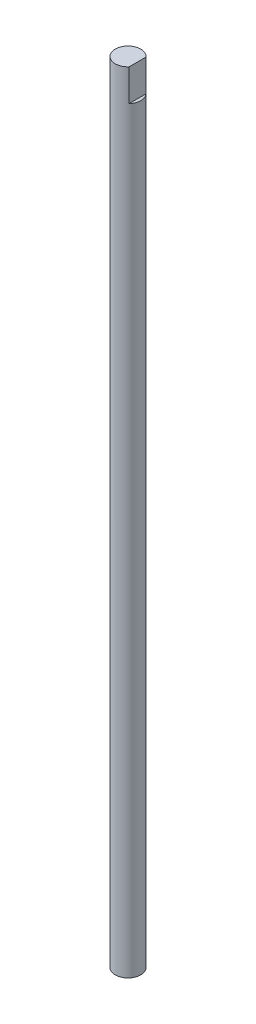
SolidWorks part; units mm, degrees
material "Q235"
ref_plane "Front" through (0, 0, 0) normal (0, 0, 1) x (1, 0, 0)
ref_plane "Top" through (0, 0, 0) normal (0, 1, 0) x (1, 0, 0)
ref_plane "Right" through (0, 0, 0) normal (1, 0, 0) x (0, 0, -1)
sketch "Sketch1" plane through (0, 0, 0) normal (0, 1, 0) x (1, 0, 0)
  circle A0 centre (0, 0) radius 8
  dimension "D1" = 16
extrude "Boss-Extrude1" add sketch "Sketch1" along normal blind 495
sketch "Sketch2" plane through (0, 0, 0) normal (0, 0, 1) x (1, 0, 0)
  line L1 (8, 475) -> (6, 475)
  line L2 (8, 475) -> (8, 495)
  line L3 (8, 495) -> (6, 495)
  line L4 (6, 475) -> (6, 495)
  line L5 (8, 495) -> (-8, 495) construction
  line L6 (8, 0) -> (8, 495) construction
  dimension "D1" = 20
  dimension "D2" = 2
extrude "Cut-Extrude1" cut sketch "Sketch2" against normal through all both and the other way through all
